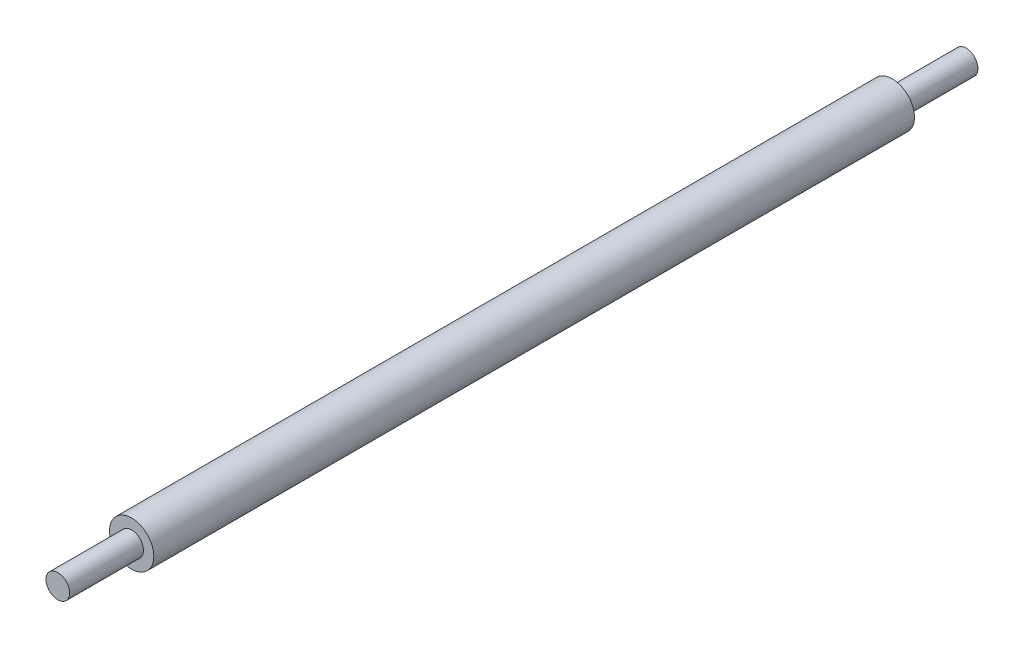
from build123d import *

# Parameters (mm, degrees)
SKETCH1_R           = 15
BOSS_EXTRUDE1_DEPTH = 257.5
SKETCH2_R           = 8
BOSS_EXTRUDE2_DEPTH = 50
BOSS_EXTRUDE3_START = 50
SKETCH3_R           = 8
BOSS_EXTRUDE3_DEPTH = 50


with BuildPart() as part:
    # Sketch1 → Boss-Extrude1 (new, symmetric)
    with BuildSketch(Plane.XY):
        Circle(SKETCH1_R)
    extrude(amount=BOSS_EXTRUDE1_DEPTH, both=True)

    # Sketch2 → Boss-Extrude2 (add)
    with BuildSketch(Plane.XY.offset(257.5)):
        Circle(SKETCH2_R)
    extrude(amount=BOSS_EXTRUDE2_DEPTH)

    # Sketch3 → Boss-Extrude3 (add)
    with BuildSketch(Plane(origin=(0, 0, -257.5), x_dir=(-1, 0, 0), z_dir=(0, 0, -1)).offset(BOSS_EXTRUDE3_START)):
        with Locations(Location((0, 0, 0), (0, 0, 180))):
            Circle(SKETCH3_R)
    extrude(amount=-BOSS_EXTRUDE3_DEPTH)


solid = part.part
